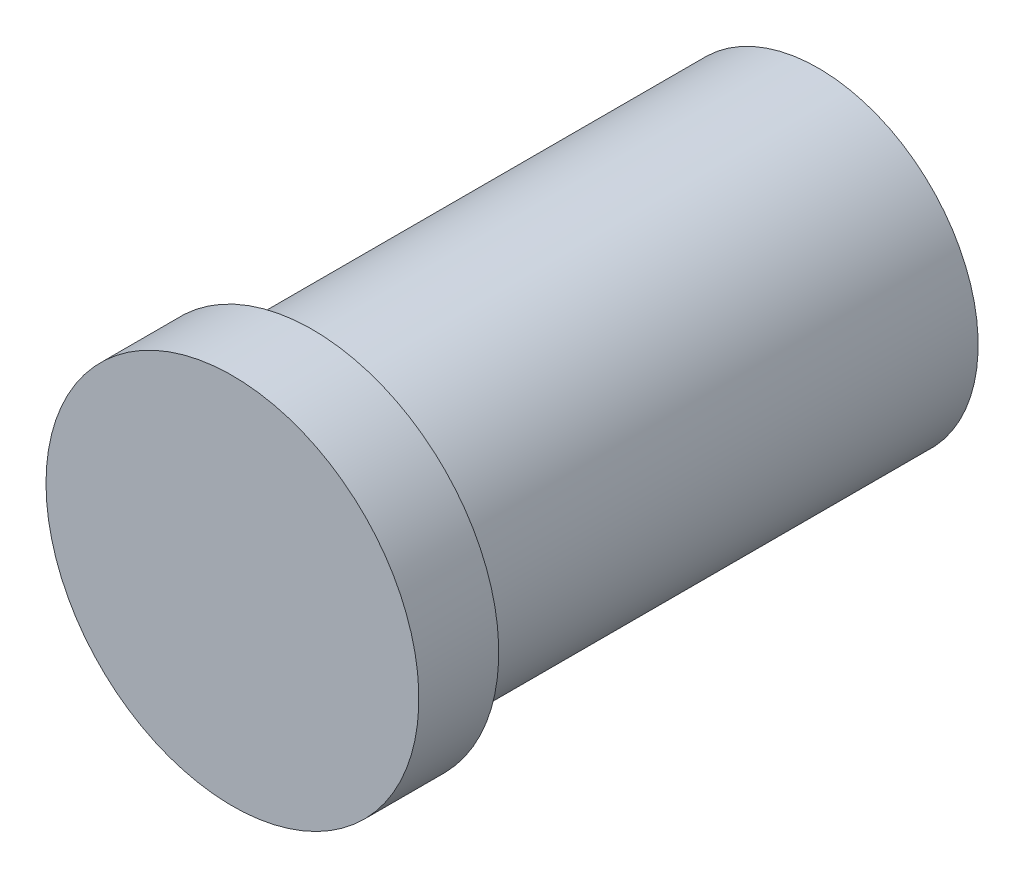
SolidWorks part; units mm, degrees
material "40Cr"
ref_plane "Front Plane" through (0, 0, 0) normal (0, 0, 1) x (1, 0, 0)
ref_plane "Top Plane" through (0, 0, 0) normal (0, 1, 0) x (1, 0, 0)
ref_plane "Right Plane" through (0, 0, 0) normal (1, 0, 0) x (0, 0, -1)
other "Configuration Table"
sketch "Sketch1" plane through (0, 0, 0) normal (0, 1, 0) x (1, 0, 0)
  line L0 (0, 0) -> (7, 0)
  line L1 (7, 0) -> (7, 3)
  line L2 (6, 22) -> (0, 22)
  line L3 (0, 22) -> (0, 0)
  line L4 (7, 3) -> (6, 3)
  line L5 (6, 3) -> (6, 22)
  dimension "D1" = 22
  dimension "D2" = 3
  dimension "D3" = 7
  dimension "D4" = 6
revolve "Revolve1" add sketch "Sketch1" angle 360 about L3
